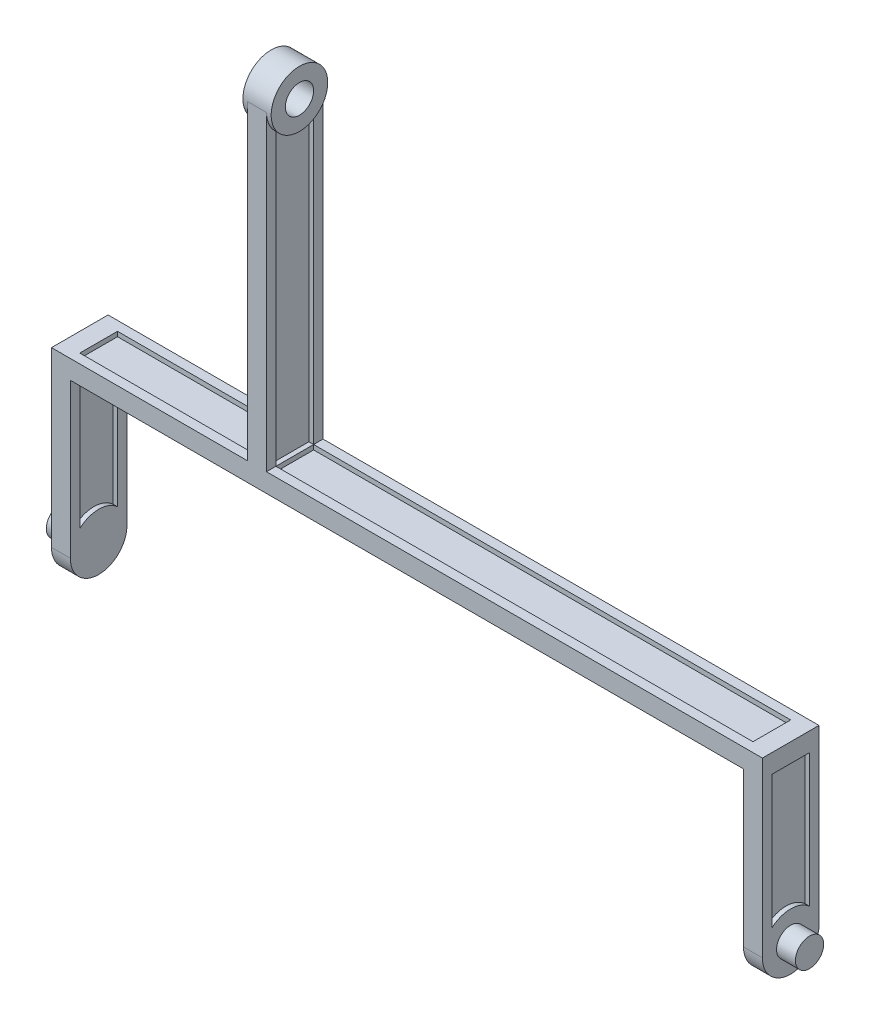
SolidWorks part; units mm, degrees
ref_plane "前视基准面" through (0, 0, 0) normal (0, 0, 1) x (1, 0, 0)
ref_plane "上视基准面" through (0, 0, 0) normal (0, 1, 0) x (1, 0, 0)
ref_plane "右视基准面" through (0, 0, 0) normal (1, 0, 0) x (0, 0, -1)
sketch "草图2" plane through (0, 0, 0) normal (1, 0, 0) x (0, 0, -1)
  circle A0 centre (0, 34.2844) radius 15
  circle A1 centre (0, 34.2844) radius 30
extrude "凸台-拉伸1" add sketch "草图2" along normal mid plane 30
sketch "草图3" plane through (0, 0, 0) normal (1, 0, 0) x (0, 0, -1)
  line L0 (-30, 34.2844) -> (-30, -315.7156)
  line L1 (-30, -315.7156) -> (30, -315.7156)
  line L2 (30, -315.7156) -> (30, 34.2844)
  circle A0 centre (0, 34.2844) radius 30 construction
  arc A1 (-30, 34.2844) -> (30, 34.2844) centre (0, 34.2844) ccw
extrude "凸台-拉伸2" add sketch "草图3" along normal mid plane 20
sketch "草图4" plane through (10, 0, 0) normal (1, 0, 0) x (0, 0, -1)
  line L1 (-30, -315.7156) -> (30, -315.7156) construction
  line L2 (-20, -315.7156) -> (-20, 11.9238)
  line L4 (20, 11.9238) -> (20, -315.7156)
  line L5 (20, -315.7156) -> (-20, -315.7156)
  arc A0 (-30, 34.2844) -> (30, 34.2844) centre (0, 34.2844) ccw construction
  circle A1 centre (0, 34.2844) radius 30 construction
  arc A2 (-20, 11.9238) -> (20, 11.9238) centre (0, 34.2844) ccw
extrude "切除-拉伸1" cut sketch "草图4" against normal blind 5
sketch "草图5" plane through (-10, 0, 0) normal (-1, 0, 0) x (0, 0, 1)
  line L0 (-20, 11.9238) -> (-20, -315.7156)
  line L1 (-20, -315.7156) -> (20, -315.7156)
  line L2 (20, -315.7156) -> (20, 11.9238)
  arc A0 (-20, 11.9238) -> (20, 11.9238) centre (0, 34.2844) ccw
extrude "切除-拉伸2" cut sketch "草图5" against normal blind 5
sketch "草图6" plane through (0, 0, 0) normal (1, 0, 0) x (0, 0, -1)
  line L1 (-30, -315.7156) -> (30, -315.7156)
  line L2 (-30, -315.7156) -> (-30, -295.7156)
  line L3 (-30, -295.7156) -> (30, -295.7156)
  line L4 (30, -315.7156) -> (30, -295.7156)
extrude "凸台-拉伸3" add sketch "草图6" against normal blind 218 and the other way blind 536
sketch "草图8" plane through (0, -295.7156, 0) normal (0, 1, 0) x (1, 0, 0)
  line L0 (-218, 30) -> (-218, -30) construction
  line L1 (-10, 20) -> (-198, 20)
  line L2 (-10, 20) -> (-10, -20)
  line L3 (-10, -20) -> (-198, -20)
  line L4 (-198, 20) -> (-198, -20)
  line L5 (10, 20) -> (516, 20)
  line L6 (10, 20) -> (10, -20)
  line L7 (10, -20) -> (516, -20)
  line L8 (516, 20) -> (516, -20)
  line L9 (536, 30) -> (536, -30) construction
  dimension "D1" = 20
  dimension "D2" = 20
extrude "切除-拉伸3" cut sketch "草图8" against normal blind 5
sketch "草图9" plane through (0, -315.7156, 0) normal (0, -1, 0) x (1, 0, 0)
  line L1 (-198, 20) -> (516, 20)
  line L2 (-198, 20) -> (-198, -20)
  line L3 (-198, -20) -> (516, -20)
  line L4 (516, 20) -> (516, -20)
extrude "切除-拉伸4" cut sketch "草图9" against normal blind 5
sketch "草图11" plane through (536, 0, 0) normal (1, 0, 0) x (0, 0, -1)
  line L3 (30, -479.2156) -> (30, -315.7156)
  line L4 (30, -315.7156) -> (-30, -315.7156)
  line L5 (-30, -479.2156) -> (-30, -315.7156)
  arc A0 (-30, -479.2156) -> (30, -479.2156) centre (0, -479.2156) ccw
extrude "凸台-拉伸4" add sketch "草图11" against normal blind 20
sketch "草图12" plane through (-218, 0, 0) normal (-1, 0, 0) x (0, 0, 1)
  line L1 (-30, -315.7156) -> (30, -315.7156)
  line L2 (-30, -315.7156) -> (-30, -479.2156)
  line L4 (30, -315.7156) -> (30, -479.2156)
  arc A0 (-30, -479.2156) -> (30, -479.2156) centre (0, -479.2156) ccw
extrude "凸台-拉伸5" add sketch "草图12" against normal blind 20
sketch "草图13" plane through (-218, 0, 0) normal (-1, 0, 0) x (0, 0, 1)
  line L1 (-20, -315.7156) -> (20, -315.7156)
  line L2 (-20, -315.7156) -> (-20, -456.8549)
  line L4 (20, -315.7156) -> (20, -456.8549)
  arc A0 (20, -456.8549) -> (-20, -456.8549) centre (0, -479.2156) ccw
extrude "切除-拉伸5" cut sketch "草图13" against normal blind 5
sketch "草图14" plane through (-198, 0, 0) normal (1, 0, 0) x (0, 0, -1)
  line L0 (-20, -456.8549) -> (-20, -315.7156)
  line L1 (-20, -315.7156) -> (20, -315.7156)
  line L2 (20, -315.7156) -> (20, -456.8549)
  arc A0 (20, -456.8549) -> (-20, -456.8549) centre (0, -479.2156) ccw
extrude "切除-拉伸6" cut sketch "草图14" against normal blind 5
sketch "草图15" plane through (536, 0, 0) normal (1, 0, 0) x (0, 0, -1)
  line L0 (-20, -456.8549) -> (-20, -315.7156)
  line L1 (-20, -315.7156) -> (20, -315.7156)
  line L2 (20, -315.7156) -> (20, -456.8549)
  arc A0 (-20, -456.8549) -> (20, -456.8549) centre (0, -479.2156) cw
extrude "切除-拉伸7" cut sketch "草图15" against normal blind 5
sketch "草图16" plane through (516, 0, 0) normal (-1, 0, 0) x (0, 0, 1)
  line L0 (-20, -456.8549) -> (-20, -315.7156)
  line L1 (-20, -315.7156) -> (20, -315.7156)
  line L2 (20, -315.7156) -> (20, -456.8549)
  arc A0 (20, -456.8549) -> (-20, -456.8549) centre (0, -479.2156) ccw
extrude "切除-拉伸8" cut sketch "草图16" against normal blind 5
sketch "草图17" plane through (536, 0, 0) normal (1, 0, 0) x (0, 0, -1)
  circle A0 centre (0, -479.2156) radius 15
extrude "凸台-拉伸6" add sketch "草图17" along normal blind 20
sketch "草图18" plane through (-218, 0, 0) normal (-1, 0, 0) x (0, 0, 1)
  circle A0 centre (0, -479.2156) radius 15.5
extrude "凸台-拉伸7" add sketch "草图18" along normal blind 20
